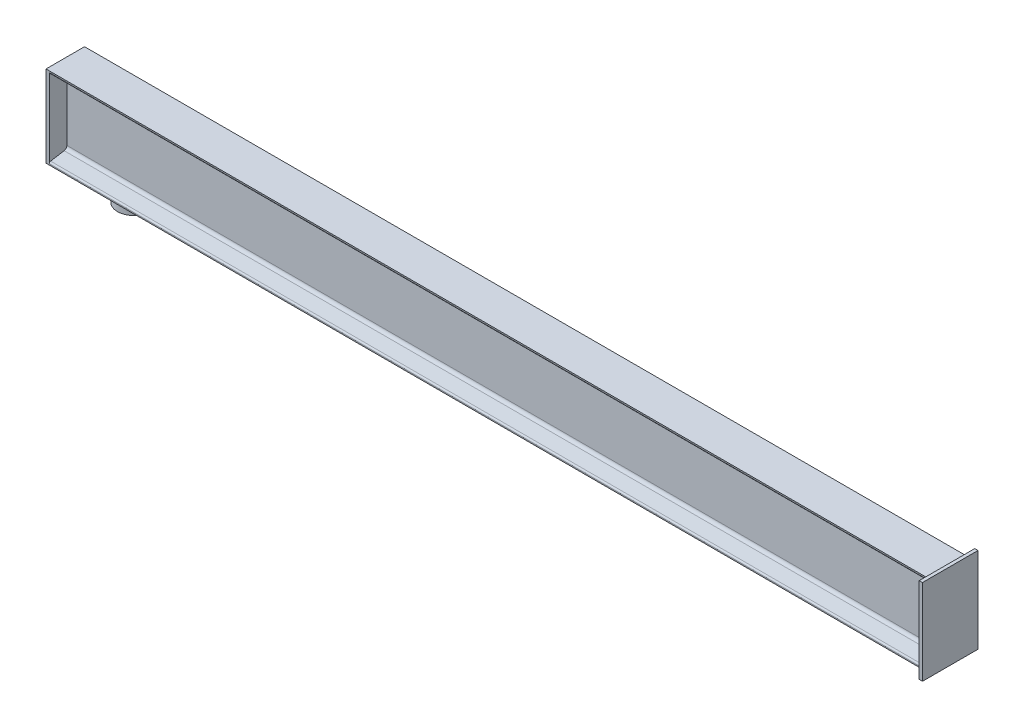
from build123d import *

# Parameters (mm, degrees)
BASE_DEPTH          = 2700
FILLET1_R           = 10
FILLET2_R           = 5
SKETCH_1_W          = 118
SKETCH_1_H          = 250
BOSS_EXTRUDE1_DEPTH = 5
SKETCH2_W           = 170
SKETCH2_H           = 262
BOSS_EXTRUDE2_DEPTH = 5
SKETCH3_R           = 50
BOSS_EXTRUDE3_DEPTH = 28


with BuildPart() as part:
    # Sketch1 → Base (new body)
    with BuildSketch(Plane(origin=(0, 0, 0), x_dir=(0, 0, -1), z_dir=(1, 0, 0))):
        Polygon((-59, 0), (59, 0), (59, 7.666666667), (5, 16.666666667), (5, 233.333333333), (59, 242.333333333), (59, 250), (-59, 250), (-59, 242.333333333), (-5, 233.333333333), (-5, 16.666666667), (-59, 7.666666667), align=None)
    extrude(amount=BASE_DEPTH)

    # Fillet1
    fillet1_edges = [part.edges().sort_by_distance(p)[0] for p in [
        (1350, 16.666666667, 5),
        (1350, 233.333333333, 5),
        (1350, 233.333333333, -5),
        (1350, 16.666666667, -5),
    ]]
    fillet(fillet1_edges, radius=FILLET1_R)

    # Fillet2
    fillet2_edges = [part.edges().sort_by_distance(p)[0] for p in [
        (1350, 7.666666667, 59),
        (1350, 242.333333333, 59),
        (1350, 242.333333333, -59),
        (1350, 7.666666667, -59),
    ]]
    fillet(fillet2_edges, radius=FILLET2_R)

    # 草图1 → Boss-Extrude1 (add, symmetric)
    with BuildSketch(Plane.ZY):
        with Locations((0, 125)):
            Rectangle(SKETCH_1_W, SKETCH_1_H)
    extrude(amount=BOSS_EXTRUDE1_DEPTH, both=True)

    # Sketch2 → Boss-Extrude2 (add, symmetric)
    with BuildSketch(Plane(origin=(2700, 0, 0), x_dir=(0, 0, -1), z_dir=(1, 0, 0))):
        with Locations((0, 125)):
            Rectangle(SKETCH2_W, SKETCH2_H)
    extrude(amount=BOSS_EXTRUDE2_DEPTH, both=True)

    # Sketch3 → Boss-Extrude3 (add)
    with BuildSketch(Plane(origin=(0, 0, 0), x_dir=(-1, 0, 0), z_dir=(0, -1, 0))):
        with Locations(Location((-205, 0, 0), (0, 0, 270))):
            Circle(SKETCH3_R)
    extrude(amount=BOSS_EXTRUDE3_DEPTH)


solid = part.part
